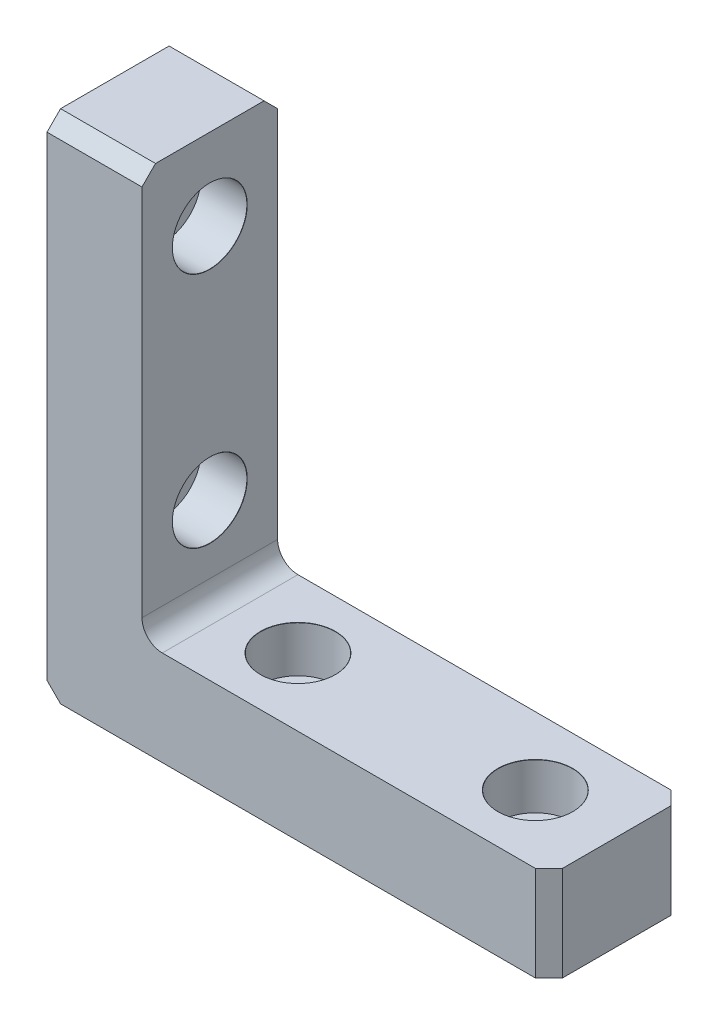
SolidWorks part; units mm, degrees
ref_plane "前视基准面" through (0, 0, 0) normal (0, 0, 1) x (1, 0, 0)
ref_plane "上视基准面" through (0, 0, 0) normal (0, 1, 0) x (1, 0, 0)
ref_plane "右视基准面" through (0, 0, 0) normal (1, 0, 0) x (0, 0, -1)
sketch "草图1" plane through (0, 0, 0) normal (0, 0, 1) x (1, 0, 0)
  line L0 (0, 0) -> (-74, 0)
  line L1 (-74, 0) -> (-74, 74)
  line L2 (-74, 74) -> (-60, 74)
  line L3 (-60, 74) -> (-60, 14)
  line L4 (-60, 14) -> (0, 14)
  line L5 (0, 14) -> (0, 0)
  dimension "D1" = 14
  dimension "D2" = 60
extrude "凸台-拉伸1" add sketch "草图1" along normal mid plane 20
fillet "圆角1" radius 3 1 edges at (-60, 14, 0)
chamfer "倒角1" distance 2 angle 45 4 edges at (0, 7, 10) (0, 7, -10) (-67, 74, 10) (-67, 74, -10)
chamfer "倒角2" distance 2 angle 45 1 edges at (-74, 0, 0)
hole_wizard "打孔尺寸(%根据)内六角圆柱头螺钉的类型1" positions "3D草图1" profile "草图2" counterbore size "M6" standard "GB" end condition up to next
sketch3d "3D草图1"
  line L0 (-60, 74, 0) -> (-60, 17, 0)
  line L1 (-60, 74, 8) -> (-60, 74, -8) construction
  line L2 (-60, 17, 10) -> (-60, 17, -10) construction
  point P0 (-60, 62, 0)
  point P2 (-60, 27, 0)
  point P11 (0, 0, 0)
  point P12 (0, 0, 0)
  dimension "D1" = 12
  dimension "D2" = 35
sketch "草图2" plane through (-60, 62, 0) normal (0, 1, 0) x (0, 0, -1)
  line L0 (0, 0) -> (0, 14)
  line L1 (0, 14) -> (3.3, 14)
  line L3 (3.3, 14) -> (3.3, 6.8)
  line L4 (5.5, 6.8) -> (3.3, 6.8)
  line L5 (5.5, 6.8) -> (5.5, 0.025)
  line L6 (5.5, 0.025) -> (5.525, 0)
  line L7 (5.525, 0) -> (0, 0)
  line L8 (-5.5, 0.025) -> (-5.525, 0) construction
  line L11 (0, -6.35) -> (0, 107.95) construction
  dimension "通孔孔直径" = 6.6
  dimension "通孔孔深度" = 14
  dimension "柱形沉头孔直径" = 11
  dimension "柱形沉头孔深度" = 6.8
  dimension "近端锥形沉头孔直径" = 11.05
  dimension "近端锥形沉头孔角度" = 90
hole_wizard "打孔尺寸(%根据)内六角圆柱头螺钉的类型2" positions "3D草图2" profile "草图4" counterbore size "M6" standard "GB" end condition up to next
sketch3d "3D草图2"
  line L0 (0, 14, 0) -> (-57, 14, 0)
  line L1 (0, 14, 8) -> (0, 14, -8) construction
  line L2 (-57, 14, -10) -> (-57, 14, 10) construction
  point P0 (-12, 14, 0)
  point P2 (-47, 14, 0)
  point P12 (-18.548, 14, 0)
  point P13 (-48.9237, 14, 0)
  point P14 (-12, 14, -2.247)
  point P15 (-40.3615, 14, 0)
  dimension "D1" = 12
  dimension "D2" = 35
sketch "草图4" plane through (-12, 14, 0) normal (1, 0, 0) x (0, 0, 1)
  line L0 (0, 0) -> (0, 14)
  line L1 (0, 14) -> (3.3, 14)
  line L3 (3.3, 14) -> (3.3, 6.8)
  line L4 (5.5, 6.8) -> (3.3, 6.8)
  line L5 (5.5, 6.8) -> (5.5, 0.025)
  line L6 (5.5, 0.025) -> (5.525, 0)
  line L7 (5.525, 0) -> (0, 0)
  line L8 (-5.5, 0.025) -> (-5.525, 0) construction
  line L11 (0, -6.35) -> (0, 107.95) construction
  dimension "通孔孔直径" = 6.6
  dimension "通孔孔深度" = 14
  dimension "柱形沉头孔直径" = 11
  dimension "柱形沉头孔深度" = 6.8
  dimension "近端锥形沉头孔直径" = 11.05
  dimension "近端锥形沉头孔角度" = 90
